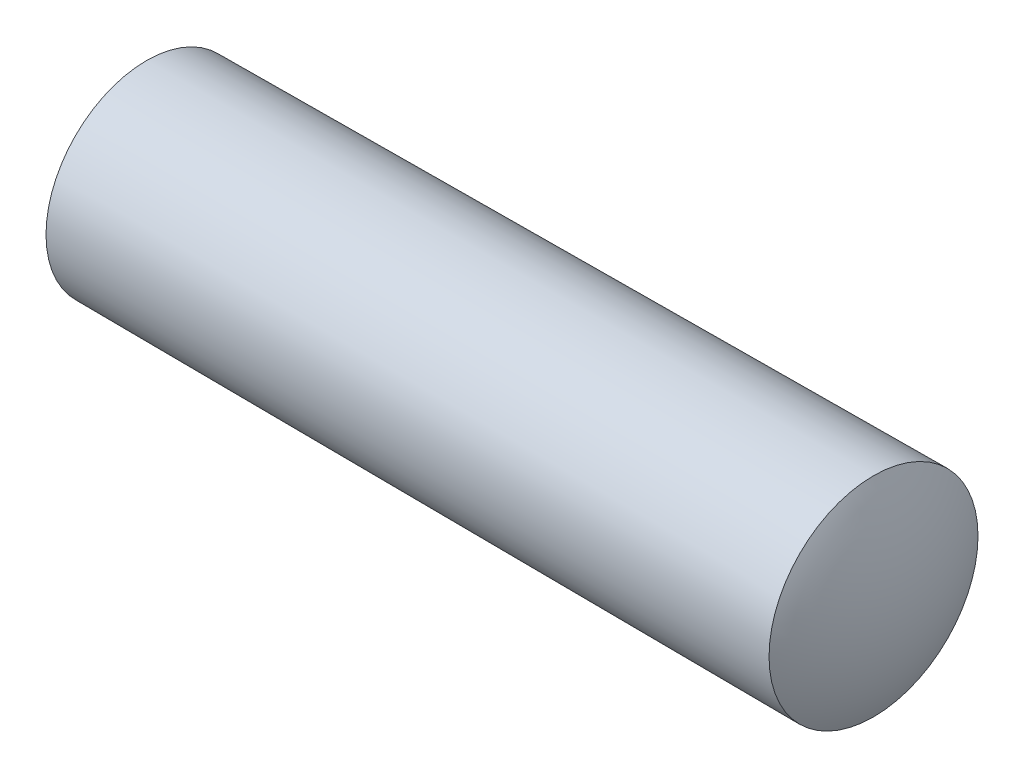
from build123d import *


with BuildPart() as part:
    # Sketch1 → Revolve1 (revolve)
    with BuildSketch(Plane.XY):
        with BuildLine():
            Line((-7, 3.872983346), (21, 4.024133344))
            ThreePointArc((21, 4.024133344), (21.746255221, 2.07326127), (22, 0))
            Line((22, 0), (-8, 0))
            ThreePointArc((-8, 0), (-7.745966692, 2), (-7, 3.872983346))
        make_face()
    revolve(axis=Axis((-8, 0, 0), (1, 0, 0)))


solid = part.part
